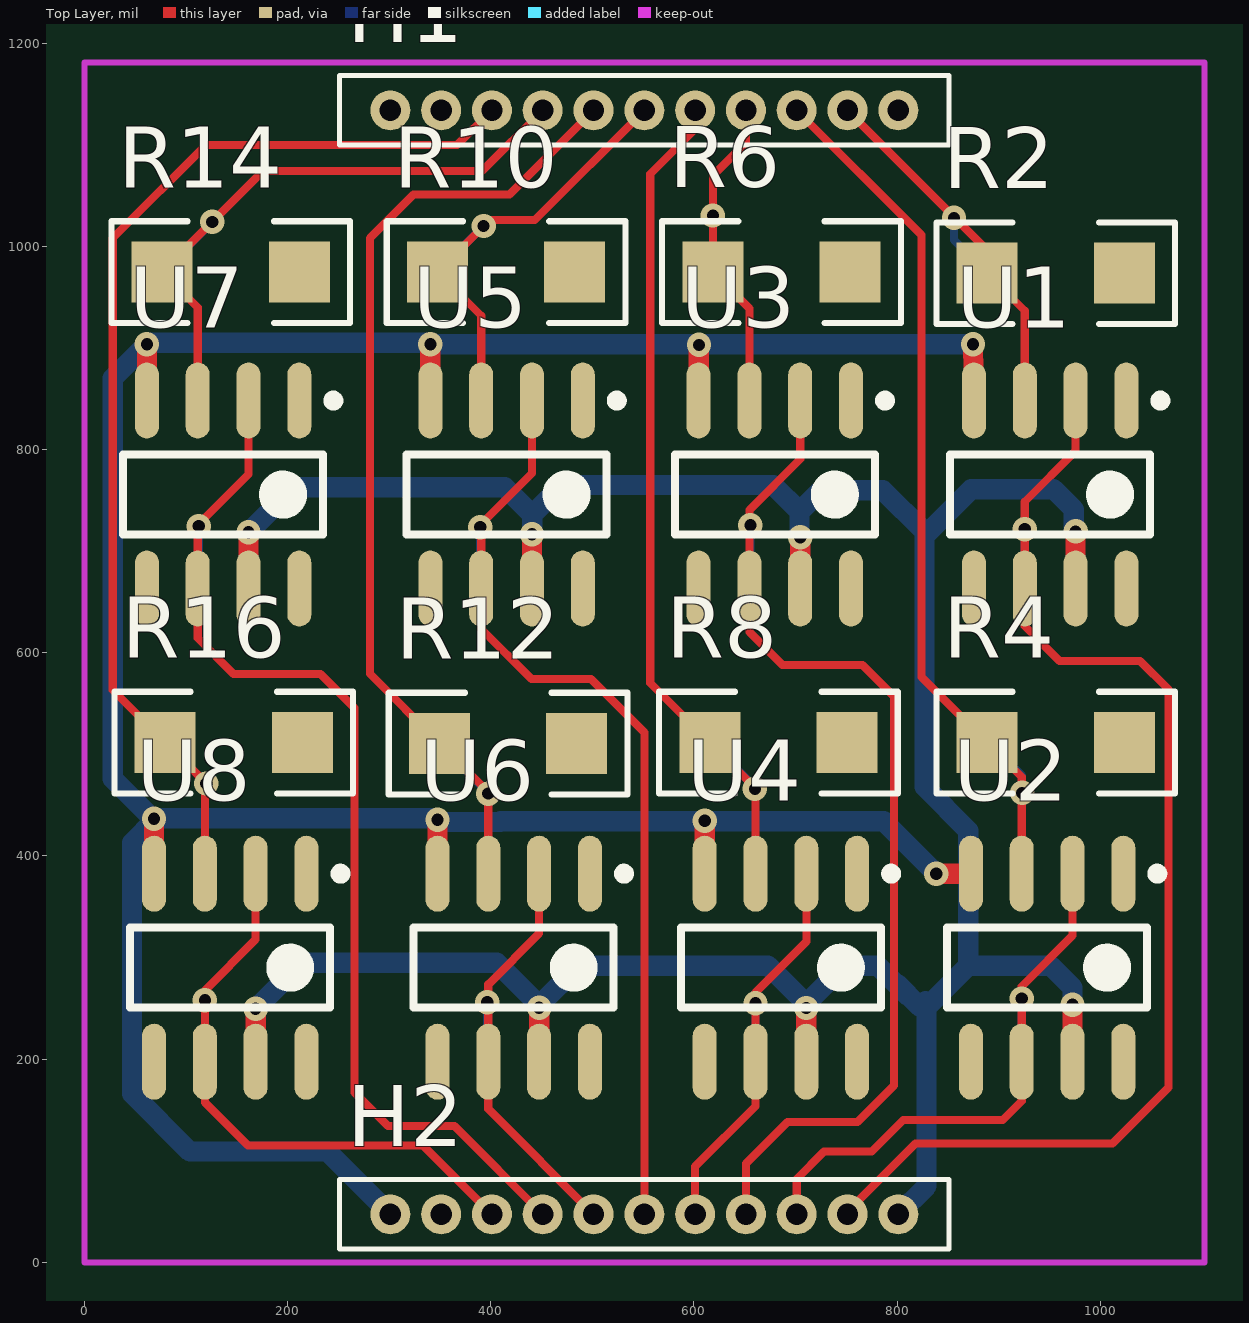
[diagram p0: Top Layer view]
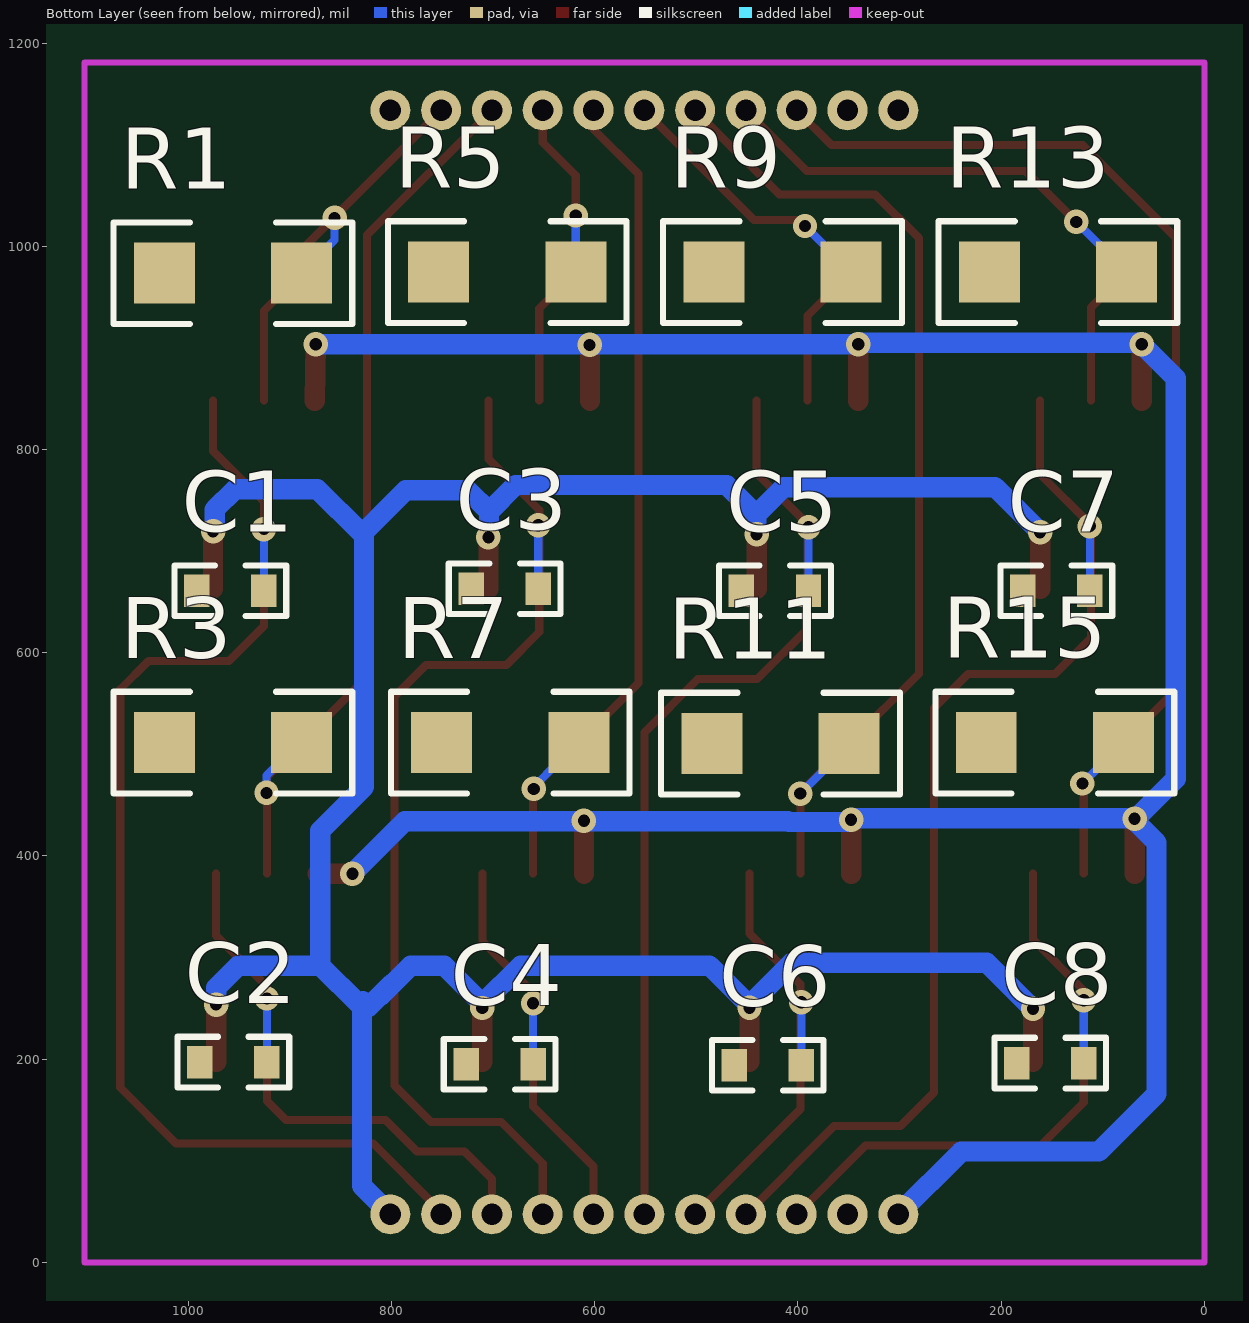
[diagram p1: Bottom Layer view, seen from below]
# Altium PCB MISC82250.PcbDoc
Units mil, origin at the board's own origin, x right, y up, seen from the top; angles counter-clockwise.
Board outline 3622.05 x 5000 mil, 2 copper layers (Top Layer, Bottom Layer); 34 components, 19 nets, 134 pads, 32 vias.
Unrouted connection lines stored in the file: 24.

## Layer stack, top to bottom (the 12.6 mil dielectric is the usual default, probably not edited)
Top Layer: signal copper 1.4
Dielectric: dielectric 12.6, FR-4, Dk 4.8
Bottom Layer: signal copper 1.4

## Board outline
-1056.37,-2673 -1056.37,2327 2565.68,2327 2565.68,-2673

## Design rules (kind name [scope] priority, off if disabled: settings)
Clearance [All] p1: gap=6
FabricationTestPointUsage TestPointUsage [All] p1: valid=0 allowmultiple=FALSE
FabricationTestpoint Testpoint [(IsPad And (OnTopLayer Or OnBottomLayer))] p1: side=3 testpointundercomponent=TRUE minsize=40 maxsize=100 preferedsize=60 minholesize=0 maxholesize=40 preferedholesize=32 testpointgrid=1 allowsidetop=TRUE allowsidebottom=TRUE usegrid=TRUE gridtolerance=0.01
HoleSize [All] p1: absolutevalues=TRUE maxlimit=150 minlimit=11.81 maxpercent=80.000 minpercent=20.000
MinimumSolderMaskSliver [All] p1: minsoldermaskwidth=0
PolygonConnect [All] p1: connectstyle=Relief reliefconductorwidth=10 reliefentries=4 polygonreliefangle="90 Angle"
RoutingVias [All] p1: holewidth=12 width=24 viastyle="Through Hole" minholewidth=12 minwidth=24 maxholewidth=12 maxwidth=24
SilkToSilkClearance [All] p1: silktosilkclearance=0
SilkscreenOverComponentPads [IsPad] p1: minsilkscreentomaskgap=0
SolderMaskExpansion [All] p1: expansion=4
Width [All] p1: maxlimit=20 minlimit=8 preferedwidth=8 minimp=50.000000 maximp=50.000000 favimp=50.000000
22 further rules are at their usual default settings.

## Components (designator, comment, footprint, x,y, rotation, side; value= is the part's Value field where it differs from the comment)
C1 "30pF" 0603 991.63,661 r180 bottom
C2 "30pF" 0603 988.63,197 r180 bottom
C3 "30pF" 0603 721.63,663 r180 bottom
C4 "30pF" 0603 726.63,195 r180 bottom
C5 "30pF" 0603 455.63,661 r180 bottom
C6 "30pF" 0603 462.63,194 r180 bottom
C7 "30pF" 0603 178.63,661 r180 bottom
C8 "30pF" 0603 184.63,196 r180 bottom
H1 "Header11" PinHeader11_1.27mm 801.18,1133.86 r180 top locked
H2 "Header11" PinHeader11_1.27mm 801.18,47.24 r180 top locked
R1 "1%" 1206 888.63,973.63 r0 bottom
R2 "1%" 1206 888.63,973.63 r0 top
R3 "1%" 1206 888.63,511.63 r0 bottom
R4 "1%" 1206 888.63,511.63 r0 top
R5 "1%" 1206 618.63,974.63 r0 bottom
R6 "1%" 1206 618.63,974.63 r0 top
R7 "1%" 1206 615.63,511.63 r0 bottom
R8 "1%" 1206 615.63,511.63 r0 top
R9 "1%" 1206 347.63,974.63 r0 bottom
R10 "1%" 1206 347.63,974.63 r0 top
R11 "1%" 1206 349.63,510.63 r0 bottom
R12 "1%" 1206 349.63,510.63 r0 top
R13 "1%" 1206 76.63,974.63 r0 bottom
R14 "1%" 1206 76.63,974.63 r0 top
R15 "1%" 1206 79.63,511.63 r0 bottom
R16 "1%" 1206 79.63,511.63 r0 top
U1 "TL061D" TL061_SOIC8 950.63,755.63 r270 top
U2 "TL061D" TL061_SOIC8 947.63,290 r270 top
U3 "TL061D" TL061_SOIC8 679.63,755.63 r270 top
U4 "TL061D" TL061_SOIC8 685.63,290 r270 top
U5 "TL061D" TL061_SOIC8 415.63,755.63 r270 top
U6 "TL061D" TL061_SOIC8 422.63,290 r270 top
U7 "TL061D" TL061_SOIC8 136.63,755.63 r270 top
U8 "TL061D" TL061_SOIC8 143.63,290 r270 top

## Footprints (in the part's own frame and the unit in brackets; to place one, negate y for a bottom-side part, rotate by r counter-clockwise, add the part's x,y. Pads: shape width x height; smd on the part's side, far side on the other; paste and mask are expansions set on the pad)
0603 [mil]
  rect 25x32 smd: 1(0,0) 2(66,0)
  silkscreen extent -22,-25 88,25
1206 [mil]
  rect 60x60 smd: 1(0,0) 2(135,0)
  silkscreen extent -50,-50 185,50
PinHeader11_1.27mm [mm]
  round 1 hole 0.533: 1(0,0) 2(1.27,0) 3(2.54,0) 4(3.81,0) 5(5.08,0) 6(6.35,0) 7(7.62,0) 8(8.89,0) 9(10.16,0) 10(11.43,0) 11(12.7,0)
  silkscreen extent -1.27,-0.87 13.97,0.87
TL061_SOIC8 [mm]
  oval 1.9x0.6 smd: 1(-2.35,1.905) 2(-2.35,0.635) 3(-2.35,-0.635) 4(-2.35,-1.905) 5(2.35,-1.905) 6(2.35,-0.635) 7(2.35,0.635) 8(2.35,1.905)
  silkscreen extent -2.47,-2.5 1,2.88

## Part data
C1 C2 C3 C4 C5 C6 C7 C8: library part CAP, "Capacitor"
R1 R2 R3 R4 R5 R6 R7 R8 R9 R10 R11 R12 R13 R14 R15 R16: library part ProE260.TMP_300K_25

## Via types
v1: diameter 24, hole 12, Top Layer to Bottom Layer, 32 vias

## Nets (pads, with @x,y where several pads share a name; then routed paths per layer and width w, separated by ;. In a path a pad name is that pad's centre, name@x,y a point inside that pad or via, vN(x,y) a via of type N, cw(c..) or ccw(c..) an arc to the next point about the centre after c; other vN are vias at no path point)
+15V: H2.1 U1.7 U2.7 U3.7 U4.7 U5.7 U6.7 U7.7 U8.7 | length 3040.2
  Top Layer w20: U7.7 v1(161.63,718.63) ; U8.7 v1(168.63,249.63) ; U5.7 v1(440.63,716.63) ; U6.7 v1(447.63,250.63) ; U3.7 v1(704.63,713.63) ; U4.7 v1(710.63,250.37) ; U2.7 v1(972.63,253.63) ; U1.7 v1(975.63,719.37)
  Bottom Layer w20: v1(161.63,718.63) 206,763 414,763 441,736 ; v1(168.63,249.63) 214,295 406,295 448,253 487,292 673,292 v1@710,255 ; v1@441,716.63 441,736 ; v1@704,714 704,739 ; v1@711,255 748,292 781,292 810,263 ; 800,274 822.5,251.5 828,257 ; H2.1 829,75.06 829,256 831.5,253.5 870,292 ; 827,720 827,719 ; 829,717 827,719 ; 830,718 873,761 954,761 974,741 v1@974,719 ; v1(972.63,253.63) 972.63,270.37 951,292 870,292 ; 441,736 470,765 678,765 704,739 ; 704,739 725,760 786,760 827,719 ; 827,719 827,468 870,425 870,292
-15V: H2.11 U1.4 U2.4 U3.4 U4.4 U5.4 U6.4 U7.4 U8.4 | length 3092
  Top Layer w20: U7.4 v1(61.63,903.63) ; U8.4 v1(68.63,436.63) ; U5.4 v1(340.63,903.63) ; U6.4 v1(347.63,435.63) ; U3.4 604.63,899.63 605,900 v1(605,903) ; U4.4 v1(610.63,434.63) ; v1(838.52,382.52) U2.4 ; v1(874.63,903.63) U1.4
  Bottom Layer w20: v1@61,903 28,870 28,476 69,435 47,413 47,166 104,109 239.43,109 H2.11 ; v1@61,905 342,905 347.37,903.63 v1(874.63,903.63) ; v1@72,437 v1@347.63,437 ; v1@351.63,433.37 409.23,433.37 ; 409.86,434 787.04,434 v1(838.52,382.52)
AGND: C1.1 C2.1 C3.1 C4.1 C5.1 C6.1 C7.1 C8.1 H2.10 R1.2 R2.2 R3.2 R4.2 R5.2 R6.2 R7.2 R8.2 R9.2 R10.2 R11.2 R12.2 R13.2 R14.2 R15.2 R16.2
I1_AD: H1.2 R1.1 R2.1 U1.3 | length 403.1
  Top Layer w8: H1.2 R2.1@888.63,996.41 ; R2.1 925.63,936.63 U1.3
  Bottom Layer w8: v1(856,1028) 856,1006.26 R1.1
I2_AD: H1.3 R3.1 R4.1 U2.3 | length 871.7
  Top Layer w8: H1.3 824,1011.04 824,576.26 R4.1 922.63,477.63 v1@922.63,462 ; U2.3 v1@922.63,462 ; v1(923,462) v1@922.63,462
  Bottom Layer w8: R3.1@915,487 923,479 v1(923,462)
I3_AD: H1.4 R5.1 R6.1 U3.3 | length 369.8
  Top Layer w8: H1.4 651.18,1102.18 618.63,1069.63 R6.1 654.63,938.63 U3.3
  Bottom Layer w8: R5.1 v1(618.63,1030.37)
I4_AD: H1.5 R7.1 R8.1 U4.3 | length 849.4
  Top Layer w8: H1.5 601.18,1115.18 557,1071 557,570.26 R8.1 v1@660.63,466.63 ; v1(660,466) v1@660.63,466.63 ; U4.3 v1@660.63,466.63
  Bottom Layer w8: R7.1@636,492 660,468 v1(660,466)
I5_AD: H1.6 R9.1 R10.1 U5.3 | length 478
  Top Layer w8: U5.3 390.63,931.63 R10.1 399,1026 443.32,1026 H1.6
  Bottom Layer w8: R9.1 v1(393,1020)
I6_AD: H1.7 R11.1 R12.1 U6.3 | length 990
  Top Layer w8: U6.3 v1(397.63,461.37) 397.63,462.63 R12.1 281,579.26 281,1008 324,1051 418.32,1051 H1.7
  Bottom Layer w8: R11.1@368,493 368,491 v1(397.63,461.37)
I7_AD: H1.8 R13.1 R14.1 U7.3 | length 651.3
  Top Layer w8: U7.3 111.63,939.63 R14.1 176,1074 391.32,1074 H1.8
  Bottom Layer w8: R13.1 v1(126,1024)
I8_AD: H1.9 R15.1 R16.1 U8.3 | length 1145.4
  Top Layer w8: U8.3 118.63,472.63 R16.1 28,563.26 28,1008 119.61,1099.61 366.93,1099.61 H1.9
  Bottom Layer w8: R15.1 v1(120,471.26)
U1_AD: C1.2 H2.2 U1.2 U1.6 | length 1231.5
  Top Layer w8: H2.2 751.18,50.18 818,117 1012,117 1067,172 1067,564 1039,592 960,592 925.63,626.37 U1.6 925.63,748.63 975.63,798.63 U1.2
  Bottom Layer w8: C1.2 v1(925.63,721.63)
U2_AD: C2.2 H2.3 U2.2 U2.6 | length 595.3
  Top Layer w8: H2.3 701.18,82.18 728,109 775,109 806,140 904,140 922.63,158.63 U2.6 922.63,271.63 972.63,321.63 U2.2
  Bottom Layer w8: C2.2 v1(922.63,259.63)
U3_AD: C3.2 H2.4 U3.2 U3.6 | length 1090.1
  Top Layer w8: H2.4 651.18,97.18 692,138 761,138 797,174 797,557 766,588 687,588 654.63,620.37 U3.6 654.63,740.63 704.63,790.63 U3.2
  Bottom Layer w8: C3.2 v1(655.63,725.37)
U4_AD: C4.2 H2.5 U4.2 U4.6 | length 440.6
  Top Layer w8: H2.5 601.18,94.18 660.63,153.63 U4.6 660.63,265.63 710.63,315.63 U4.2
  Bottom Layer w8: C4.2 v1(660.63,255)
U5_AD: C5.2 H2.6 U5.2 U5.6 | length 985.1
  Top Layer w8: U5.2 440.63,776.63 390.63,726.63 U5.6 390.63,623.37 440,574 498.63,574 551.18,521.45 H2.6
  Bottom Layer w8: C5.2 v1(389.63,723.63)
U6_AD: C6.2 H2.7 U6.2 U6.6 | length 460.9
  Top Layer w8: U6.2 447.63,323.63 397.63,273.63 U6.6 397.63,150.8 H2.7
  Bottom Layer w8: C6.2 v1(396.63,256)
U7_AD: C7.2 H2.8 U7.2 U7.6 | length 1114.4
  Top Layer w8: U7.2 161.63,775.63 111.63,725.63 U7.6 111.63,614.37 147,579 232.63,579 266,545.63 266,167 299,134 364.43,134 H2.8
  Bottom Layer w8: C7.2 v1(112.63,724.63)
U8_AD: C8.2 H2.9 U8.2 U8.6 | length 636
  Top Layer w8: U8.2 168.63,317.63 118.63,267.63 U8.6 118.63,157.37 161,115 333.43,115 H2.9
  Bottom Layer w8: C8.2 v1(118.63,258)
pads on no net: H1.1 H1.10 H1.11 U1.1 U1.5 U1.8 U2.1 U2.5 U2.8 U3.1 U3.5 U3.8 U4.1 U4.5 U4.8 U5.1 U5.5 U5.8 U6.1 U6.5 U6.8 U7.1 U7.5 U7.8 U8.1 U8.5 U8.8

## Keep-outs
Keep-Out Layer:
  lines w6: 0,0 0,1181.1 1102.36,1181.1 1102.36,0 0,0

## Silkscreen, mask and mechanical layers (free items; w line width, h text height)
Mechanical 1:
  the board outline again, w10